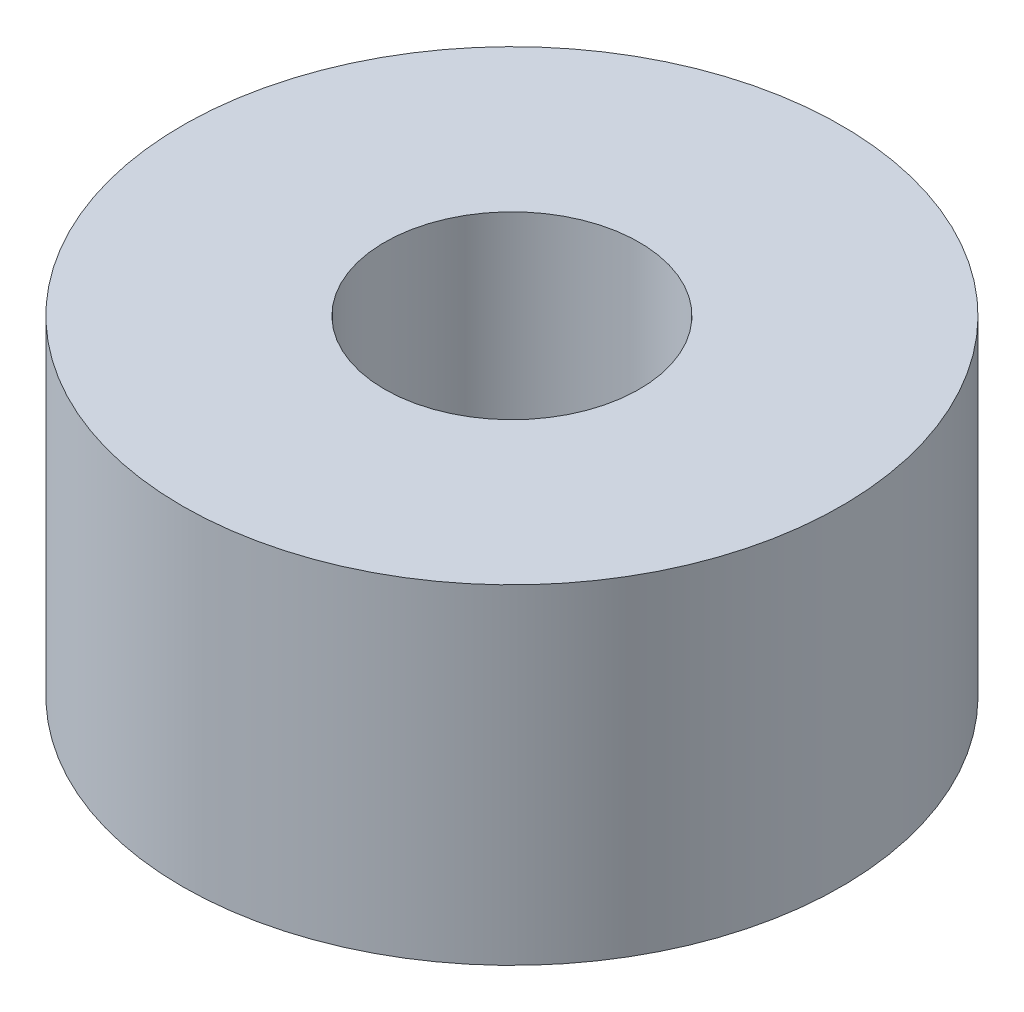
from build123d import *

# Parameters (mm, degrees)
SKETCH1_R              = 11
SKETCH1_R_2            = 4
BOSS_EXTRUDE1_DEPTH    = 11
M10_TAPPED_HOLE1_D     = 8.5
M10_TAPPED_HOLE1_DEPTH = 24.5
M10_TAPPED_HOLE1_TIP   = 2.553657631


with BuildPart() as part:
    # Sketch1 → Boss-Extrude1 (new body)
    with BuildSketch(Plane(origin=(0, 0, 0), x_dir=(1, 0, 0), z_dir=(0, 1, 0))):
        with Locations(Location((0, 0, 0), (0, 0, 270))):
            Circle(SKETCH1_R)
        with Locations(Location((0, 0, 0), (0, 0, 270))):
            Circle(SKETCH1_R_2, mode=Mode.SUBTRACT)
    extrude(amount=BOSS_EXTRUDE1_DEPTH)

    # M10 Tapped Hole1
    with Locations(Plane(origin=(0, 11, 0), x_dir=(1, 0, 0), z_dir=(0, 1, 0))):
        with Locations((0, 0)):
            Hole(M10_TAPPED_HOLE1_D / 2, depth=M10_TAPPED_HOLE1_DEPTH)
            with Locations((0, 0, -(M10_TAPPED_HOLE1_DEPTH + M10_TAPPED_HOLE1_TIP / 2))):  # 118° drill point
                Cone(0, M10_TAPPED_HOLE1_D / 2, M10_TAPPED_HOLE1_TIP, mode=Mode.SUBTRACT)


solid = part.part
